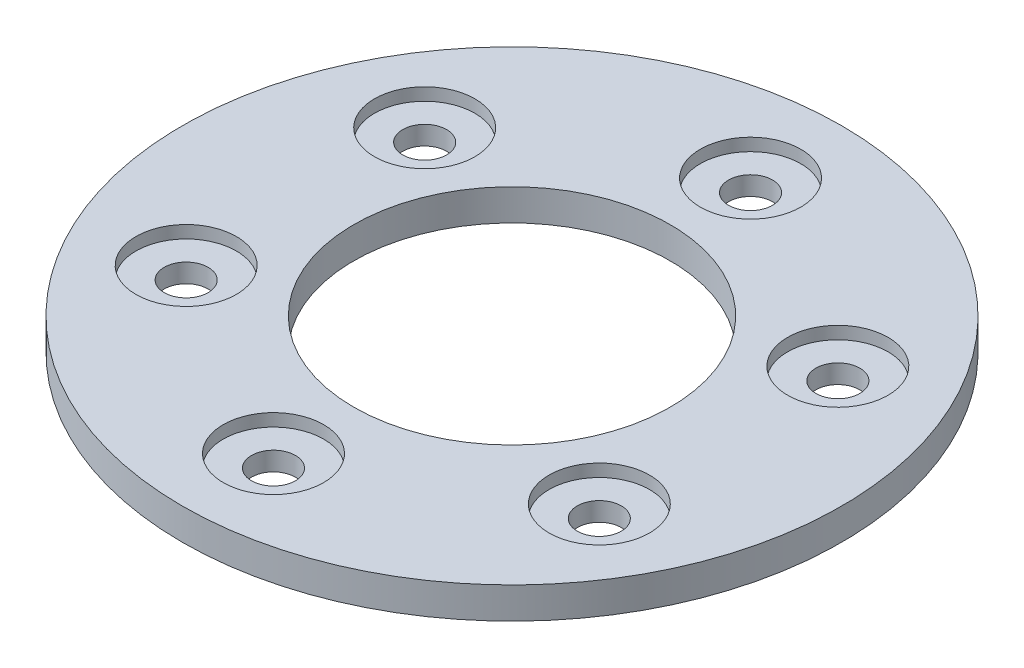
SolidWorks part; units mm, degrees
material "7075-T6 (SN)"
ref_plane "Front Plane" through (0, 0, 0) normal (0, 0, 1) x (1, 0, 0)
ref_plane "Top Plane" through (0, 0, 0) normal (0, 1, 0) x (1, 0, 0)
ref_plane "Right Plane" through (0, 0, 0) normal (1, 0, 0) x (0, 0, -1)
sketch "Sketch1" plane through (0, 0, 0) normal (0, 1, 0) x (1, 0, 0)
  circle A0 centre (0, 0) radius 12.6
  circle A1 centre (0, 0) radius 26.25
  dimension "D1" = 52.5
  dimension "D2" = 25.2
extrude "Boss-Extrude1" add sketch "Sketch1" along normal blind 4
sketch "Sketch2" plane through (0, 4, 0) normal (0, 1, 0) x (1, 0, 0)
  circle A0 centre (0, 0) radius 14.25
  circle A1 centre (0, 0) radius 35
  dimension "D1" = 28.5
  dimension "D2" = 70
extrude "Cut-Extrude1" cut sketch "Sketch2" against normal blind 1.5
sketch "Sketch4" plane through (0, 2.5, 0) normal (0, 1, 0) x (1, 0, 0)
  line L0 (0, 0) -> (-50000, 0) construction
  line L1 (0, 0) -> (0, 50000) construction
  circle A0 centre (0, 0) radius 19 construction
  circle A2 centre (0, 19) radius 1.75
  dimension "D1" = 38
  dimension "D2" = 3.5
extrude "Cut-Extrude2" cut sketch "Sketch4" against normal blind 10
pattern_circular "CirPattern1" count 6 over 360 about axis through (0, 0, 0) along (0, 1, 0) of "Cut-Extrude2"
sketch "Sketch5" plane through (0, 2.5, 0) normal (0, 1, 0) x (1, 0, 0)
  circle A0 centre (0, 19) radius 4
  dimension "D1" = 8
extrude "Cut-Extrude3" cut sketch "Sketch5" against normal blind 1
pattern_circular "CirPattern2" count 6 over 360 about axis through (0, 0, 0) along (0, 1, 0) of "Cut-Extrude3"
chamfer "Chamfer1" distance 0.5 angle 45 1 edges at (0, 4, 14.25)
sketch "Sketch6" plane through (0, 4, 0) normal (0, 1, 0) x (1, 0, 0)
  circle A0 centre (0, 0) radius 14.25
extrude "Cut-Extrude4" cut sketch "Sketch6" against normal up to surface (1.5 mm away) up to face at (-12.9904, 2.5, -7.5)
